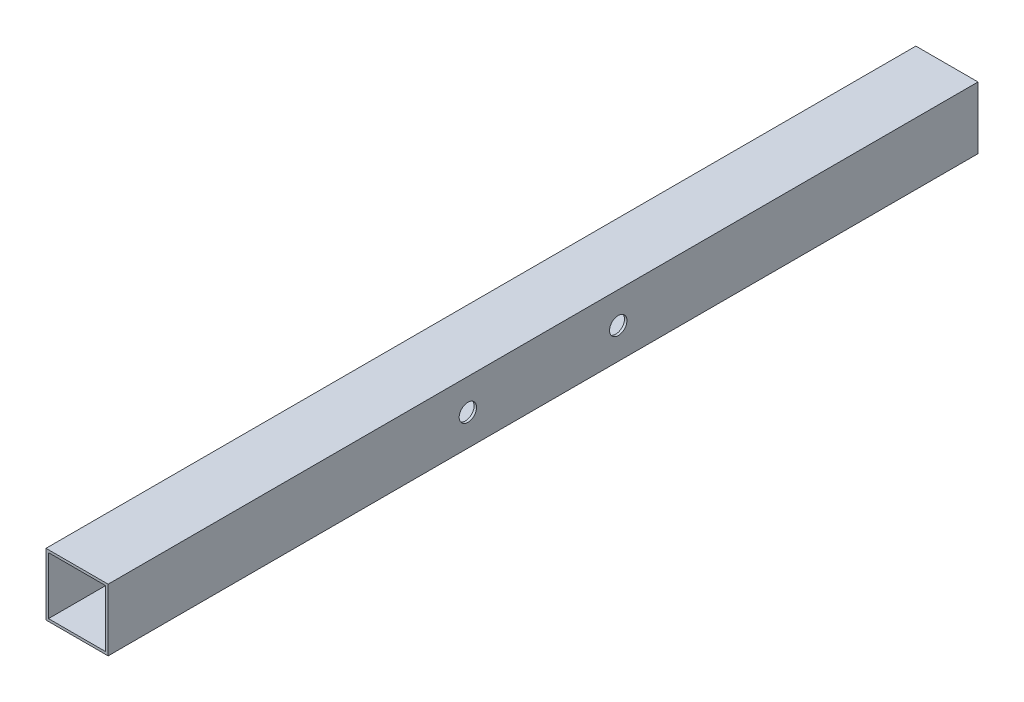
SolidWorks part; units mm, degrees
material "AISI 304"
ref_plane "Front Plane" through (0, 0, 0) normal (0, 0, 1) x (1, 0, 0)
ref_plane "Top Plane" through (0, 0, 0) normal (0, 1, 0) x (1, 0, 0)
ref_plane "Right Plane" through (0, 0, 0) normal (1, 0, 0) x (0, 0, -1)
sketch "Sketch1" plane through (0, 0, 0) normal (0, 0, 1) x (1, 0, 0)
  line L1 (-25, -25) -> (25, -25)
  line L2 (-25, -25) -> (-25, 25)
  line L3 (-25, 25) -> (25, 25)
  line L4 (25, -25) -> (25, 25)
  line L5 (-25, -25) -> (25, 25) construction
  line L6 (-25, 25) -> (25, -25) construction
  line L7 (-23, -23) -> (23, -23)
  line L8 (-23, -23) -> (-23, 23)
  line L9 (-23, 23) -> (23, 23)
  line L10 (23, -23) -> (23, 23)
  line L11 (-23, -23) -> (23, 23) construction
  line L12 (-23, 23) -> (23, -23) construction
  point P0 (0, 0)
  point P6 (0, 0)
  dimension "D1" = 50
  dimension "D2" = 50
  dimension "D3" = 46
  dimension "D4" = 46
extrude "Boss-Extrude1" add sketch "Sketch1" along normal blind 700
sketch "Sketch2" plane through (-25, 0, 0) normal (-1, 0, 0) x (0, 0, 1)
  line L0 (350, 25) -> (350, -132.5751) construction
  line L1 (700, 25) -> (0, 25) construction
  line L2 (0, 0) -> (604.8974, 0) construction
  circle A0 centre (289.5, 0) radius 7
  circle A1 centre (410.5, 0) radius 7
  dimension "D1" = 14
  dimension "D2" = 121
extrude "Cut-Extrude1" cut sketch "Sketch2" against normal through all
